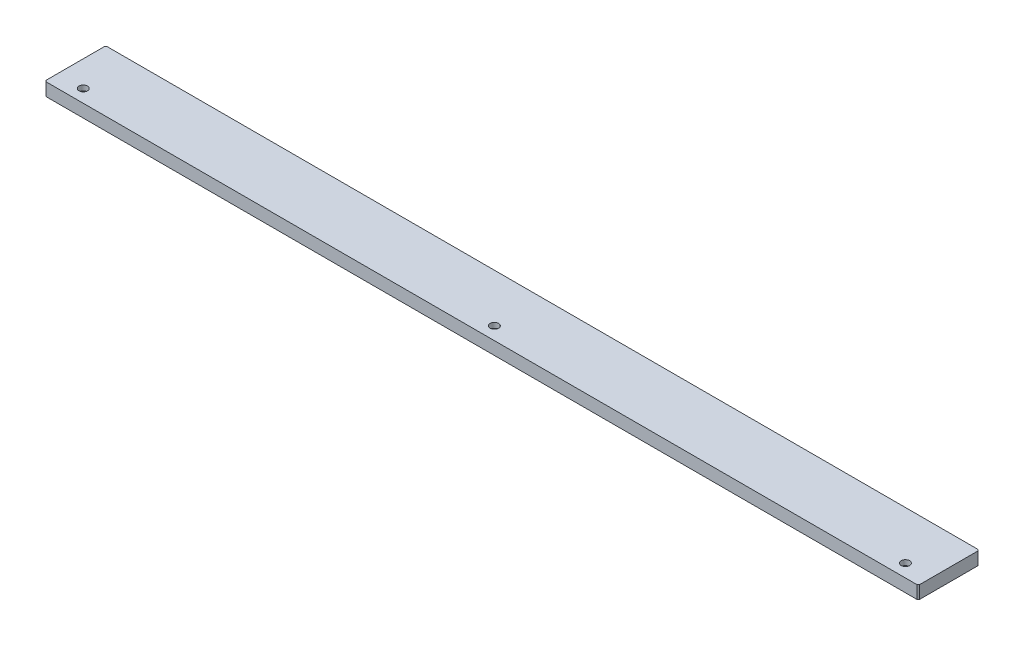
SolidWorks part; units mm, degrees
material "A6061"
ref_plane "前基準面" through (0, 0, 0) normal (0, 0, 1) x (1, 0, 0)
ref_plane "上基準面" through (0, 0, 0) normal (0, 1, 0) x (1, 0, 0)
ref_plane "右基準面" through (0, 0, 0) normal (1, 0, 0) x (0, 0, -1)
sketch "草图1" plane through (0, 0, 0) normal (0, 1, 0) x (1, 0, 0)
  line L1 (-340, -23.75) -> (340, -23.75)
  line L2 (-340, -23.75) -> (-340, 23.75)
  line L3 (-340, 23.75) -> (340, 23.75)
  line L4 (340, -23.75) -> (340, 23.75)
  line L5 (-340, -23.75) -> (340, 23.75) construction
  line L6 (-340, 23.75) -> (340, -23.75) construction
  point P0 (0, 0)
  dimension "D1" = 680
  dimension "D2" = 47.5
extrude "凸台-拉伸1" add sketch "草图1" along normal mid plane 10
chamfer "倒角1" distance 1 angle 45 4 edges at (-340, 0, 23.75) (-340, 0, -23.75) (340, 0, -23.75) (340, 0, 23.75)
hole_wizard "打孔尺寸(%根据)内六角圆柱头螺钉的类型1" positions "草图2" profile "草图3" counterbore size "M6" standard "GB" end condition through all
sketch "草图2" plane through (0, -5, 0) normal (0, -1, 0) x (-1, 0, 0)
  line L0 (-339, 23.75) -> (339, 23.75) construction
  point P0 (-320, -13.75)
  point P5 (0, -13.75)
  point P6 (320, -13.75)
  dimension "D2" = 320
  dimension "D3" = 37.5
  dimension "D1" = 3
sketch "草图3" plane through (320, -5, 13.75) normal (1, 0, 0) x (0, 0, -1)
  line L0 (0, 0) -> (0, 10)
  line L1 (0, 10) -> (3.3, 10)
  line L3 (3.3, 10) -> (3.3, 6)
  line L4 (3.3, 6) -> (5.5, 6)
  line L5 (5.5, 6) -> (5.5, 0)
  line L7 (5.5, 0) -> (0, 0)
  line L11 (0, -6.35) -> (0, 107.95) construction
  dimension "通孔孔直径" = 6.6
  dimension "通孔孔深度" = 10
  dimension "柱形沉头孔直径" = 11
  dimension "柱形沉头孔深度" = 6
hole_wizard "Ø4.1 (4.1) 直径孔1" positions "草图4" profile "草图5" hole size "Ø4.1" standard "GB"
sketch "草图4" plane through (0, 0, -23.75) normal (0, 0, -1) x (-1, 0, 0)
  point P0 (-320, 0)
  point P5 (-300, 0)
  point P6 (-280, 0)
  point P7 (-260, 0)
  point P8 (-240, 0)
  point P9 (-220, 0)
  point P10 (-200, 0)
  point P11 (-180, 0)
  point P12 (-160, 0)
  point P13 (-140, 0)
  point P14 (-120, 0)
  point P15 (-100, 0)
  point P16 (-80, 0)
  point P17 (-60, 0)
  point P18 (-40, 0)
  point P19 (-20, 0)
  point P20 (0, 0)
  point P21 (20, 0)
  point P22 (40, 0)
  point P23 (60, 0)
  point P24 (80, 0)
  point P25 (100, 0)
  point P26 (120, 0)
  point P27 (140, 0)
  point P28 (160, 0)
  point P30 (180, 0)
  point P31 (200, 0)
  point P32 (220, 0)
  point P33 (240, 0)
  point P34 (260, 0)
  point P35 (280, 0)
  point P41 (300, 0)
  point P42 (320, 0)
  dimension "D2" = 20
  dimension "D1" = 33
sketch "草图5" plane through (320, 0, -23.75) normal (1, 0, 0) x (0, 1, 0)
  line L0 (0, 0) -> (0, 11.2318)
  line L1 (0, 11.2318) -> (2.05, 10)
  line L2 (2.05, 10) -> (2.05, 0)
  line L5 (2.05, 0) -> (0, 0)
  line L10 (0, 11.2318) -> (-2.05, 10) construction
  line L11 (0, -6.35) -> (0, 107.95) construction
  dimension "孔直径" = 4.1
  dimension "孔深度" = 10
  dimension "导头角度" = 118
